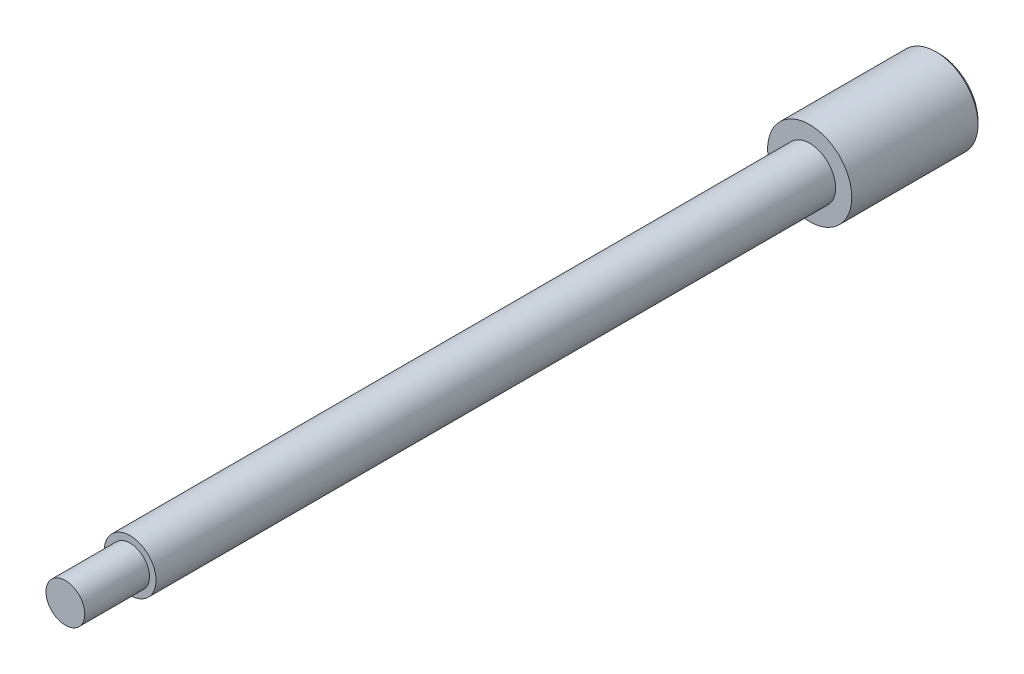
from build123d import *

# Parameters (mm, degrees)
SKETCH_1_R                = 6.5
EXTRUDE_1_DEPTH           = 20
CHAMFER_1_SIZE            = 0.5
HOLE_WIZARD_2_0_2_1_D     = 2
HOLE_WIZARD_2_0_2_1_DEPTH = 5
HOLE_WIZARD_2_0_2_1_TIP   = 0.600860619
SKETCH_8_R                = 4
EXTRUDE_2_DEPTH           = 105
SKETCH_9_R                = 3
EXTRUDE_3_DEPTH           = 10


with BuildPart() as part:
    # 草图1 → 凸台-拉伸1 (new body)
    with BuildSketch(Plane.XY):
        Circle(SKETCH_1_R)
    extrude(amount=EXTRUDE_1_DEPTH)

    # 倒角1
    chamfer_1_edges = [part.edges().sort_by_distance(p)[0] for p in [
        (-6.5, 0, 0),
    ]]
    chamfer(chamfer_1_edges, length=CHAMFER_1_SIZE)

    # Ø2.0 (2) 直径孔1
    with Locations(Plane(origin=(0, 0, 0), x_dir=(-1, 0, 0), z_dir=(0, 0, -1))):
        with Locations((-3.5, 0), (3.5, 0)):
            Hole(HOLE_WIZARD_2_0_2_1_D / 2, depth=HOLE_WIZARD_2_0_2_1_DEPTH)
            with Locations((0, 0, -(HOLE_WIZARD_2_0_2_1_DEPTH + HOLE_WIZARD_2_0_2_1_TIP / 2))):  # 118° drill point
                Cone(0, HOLE_WIZARD_2_0_2_1_D / 2, HOLE_WIZARD_2_0_2_1_TIP, mode=Mode.SUBTRACT)

    # 草图8 → 凸台-拉伸2 (add)
    with BuildSketch(Plane.XY.offset(20)):
        Circle(SKETCH_8_R)
    extrude(amount=EXTRUDE_2_DEPTH)

    # 草图9 → 凸台-拉伸3 (add)
    with BuildSketch(Plane.XY.offset(125)):
        Circle(SKETCH_9_R)
    extrude(amount=EXTRUDE_3_DEPTH)


solid = part.part
